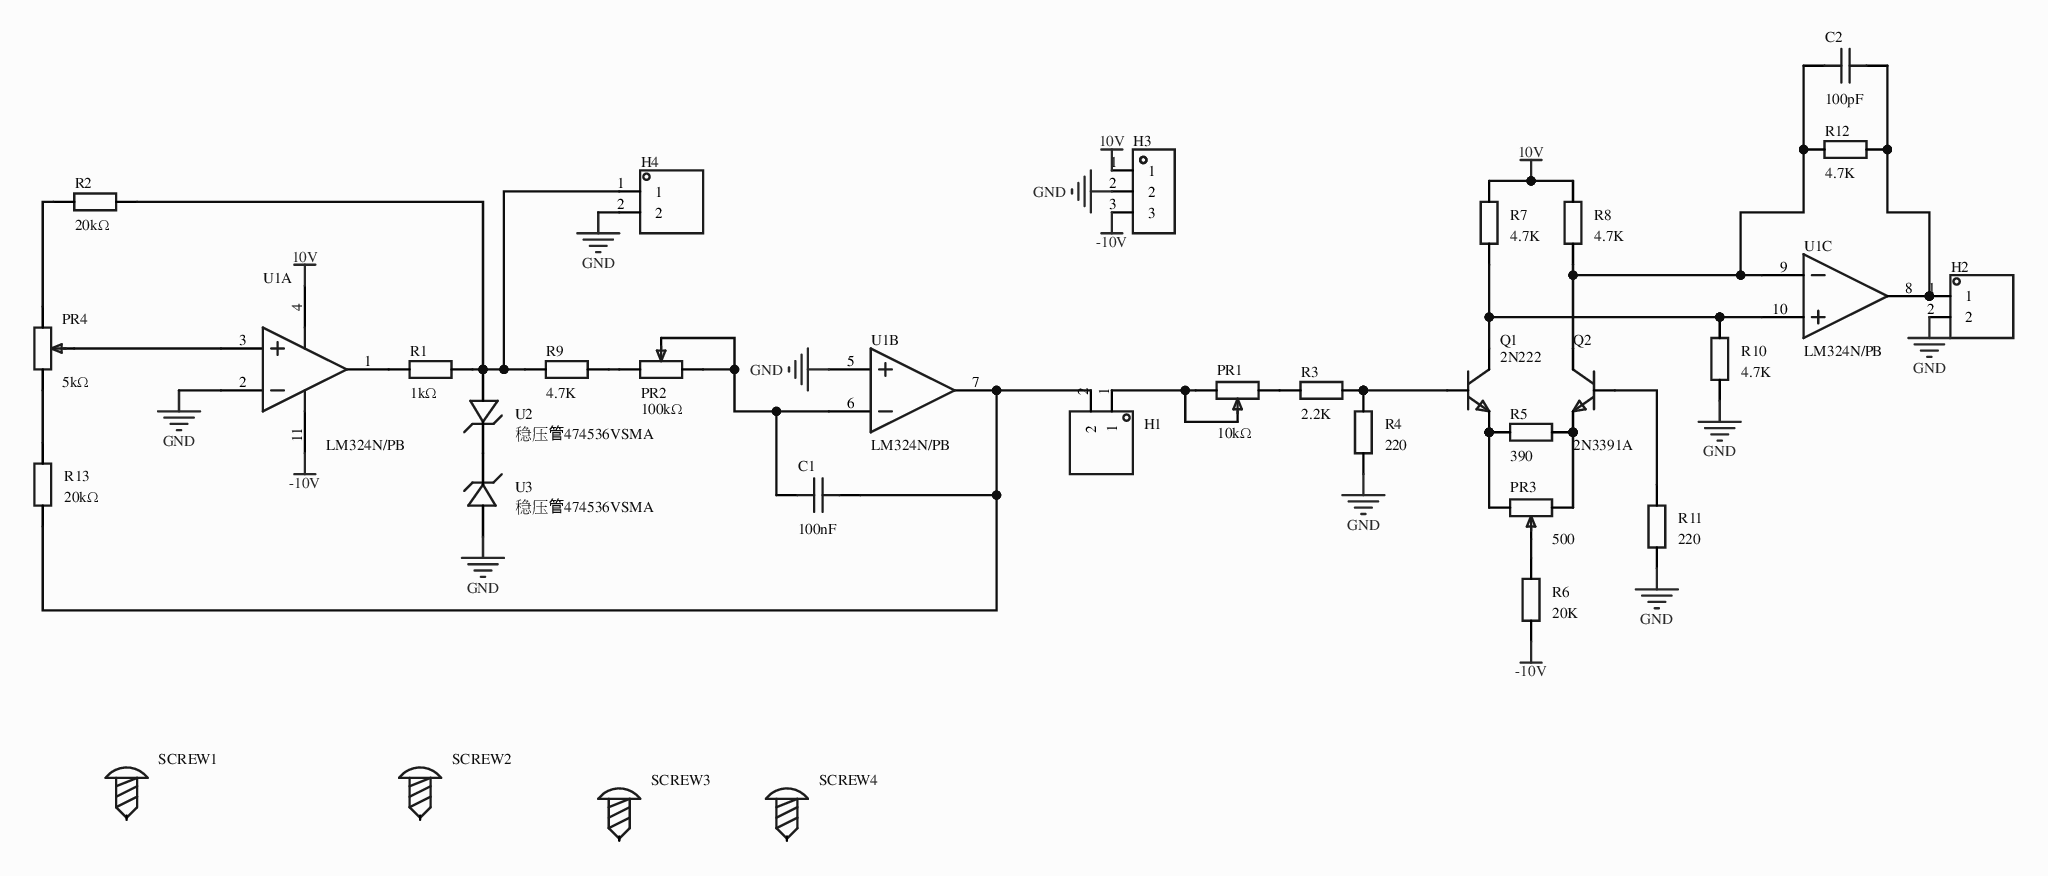
[diagram p0: MISC52119-3.schdoc]
# Altium project MISC52119-2.PrjPcb
1 sheet, 32 parts. Net scope: global (net labels, ports and power ports of the same name join across sheets).
Board file: MISC52119.pcbdoc

## Sheet MISC52119-3.schdoc
size 297 x 209 mm; Version: V1.0; @Project Name: MISC52119; @Update Date: 2026-03-23; @Create Date: 2026-03-23; @Board Name: MISC52119; @Create Time: 13:45:22; @Page Count: 1; @Page No: 1; @Schematic Name: MISC52119; @Update Time: 13:45:22; Size: A4

### Parts
C1  100nF  [C0603]
C2  100pF  [C0603]
H1  (no value)  [HDR-TH_2P-P2.54-V-M-1]
H2  (no value)  [HDR-TH_2P-P2.54-V-M-1]
H3  (no value)  [HDR-TH_3P-P2.54-V-M]
H4  (no value)  [HDR-TH_2P-P2.54-V-M-1]
PR1  10kΩ  [R_3296]
PR2  100kΩ  [R_3296]
PR3  500  [R_3296]
PR4  5kΩ  [R_3296]
Q1  2N222  [SMD_3-L3.0-W2.5_JANTXV2N2222AUB]
Q2  2N3391A  [TO-92-3_L4.9-W3.7-P1.27-L]
R1  1kΩ  [R0603]
R2  20kΩ  [R0603]
R3  2.2K  [R0603]
R4  220  [R0603]
R5  390  [R0603]
R6  20K  [R0603]
R7  4.7K  [R0603]
R8  4.7K  [R0603]
R9  4.7K  [R0603]
R10  4.7K  [R0603]
R11  220  [R0603]
R12  4.7K  [R0603]
R13  20kΩ  [R0603]
SCREW1  (no value)  [M2螺丝]
SCREW2  (no value)  [M2螺丝]
SCREW3  (no value)  [M2螺丝]
SCREW4  (no value)  [M2螺丝]
U1  LM324N/PB  [PDIP-14_L19.2-W6.6-P2.54-LS7.6-BL]  (parts A,B,C of 4)
U2  稳压管474536VSMA  [LL-41_L5.0-W2.5-RD]
U3  稳压管474536VSMA  [LL-41_L5.0-W2.5-RD]

### Nets
10V: H3.1 R7.2 R8.2 U1.4(V+)
-10V: H3.3 R6.1 U1.11(GND)
GND: H2.2 H3.2 H4.2 R4.1 R10.1 R11.1 U1.2(INA+) U1.5(INB+) U3.2(A)
NetC1_1: C1.1 H1.2 R13.2 U1.7(OUTB)
NetC1_2: C1.2 PR2.1 PR2.2 U1.6(INB-)
NetC2_1: C2.1 Q2.2(C) R8.1 R12.2 U1.9(INC-)
NetC2_2: C2.2 H2.1 R12.1 U1.8(OUTC)
NetH1_1: H1.1 PR1.1 PR1.2
NetH4_1: H4.1 R1.1 R2.1 R9.1 U2.2(A)
NetPR1_3: PR1.3 R3.1
NetPR2_3: PR2.3 R9.2
NetPR3_1: PR3.1 Q1.2(E) R5.1
NetPR3_2: PR3.2 R6.2
NetPR3_3: PR3.3 Q2.1(E) R5.2
NetPR4_1: PR4.1 R13.1
NetPR4_2: PR4.2 U1.3(INA-)
NetPR4_3: PR4.3 R2.2
NetQ1_1: Q1.1(C) R7.1 R10.2 U1.10(INC+)
NetQ1_3: Q1.3(B) R3.2 R4.2
NetQ2_3: Q2.3(B) R11.2
NetR1_2: R1.2 U1.1(OUTA)
NetU2_1: U2.1(C) U3.1(C)

Not connected (* = marked no-connect by the designer): SCREW1 1; SCREW2 1; SCREW3 1; SCREW4 1

### Library data of the parts
C1 C2 = CAP_0603: Symbol: Capacitance; 3D Model: ac125912035d415993ca9572d50418b10819f05c4eef4c71ace90d822a990e87; 3D Model Transform: 62.992,31.496,0,0,0,0,0,0,0; ConvertToPcb: yes; ModelName: C0603_L1.6-W0.8-H0.8; Device: CAP_0603; Supplier Footprint: 0603; AddInBom: yes; FootprintName: C0603
  C1: Value: 100nF
  C2: Value: 100pF
H1 H2 = HDR-M_2.54_1x2P: Symbol: 210S-1*2P L=11.6MMGold-plated black; 3D Model: 79b2e9f2d70a4d68a1b7098f27c6d4c50819f05c4eef4c71ace90d822a990e87; 3D Model Transform: 200,100,0,0,0,0,0,0,-118.11; ConvertToPcb: yes; ModelName: HDR-M-2.54_1x2; Device: HDR-M_2.54_1x2P; Supplier Part: C124375; Supplier Footprint: 插件; AddInBom: yes; FootprintName: HDR-TH_2P-P2.54-V-M-1
H3 = HDR-M_2.54_1x3P: 3D Model: bb473b6d38ff42a99216a4fcdbdcc4cb0819f05c4eef4c71ace90d822a990e87; 3D Model Transform: 300.03877,100,0,0,0,0,0,0,-118.11; AddInBom: yes; ModelName: HDR-TH_3P-P2.54-M-LI-1X3P; Symbol: HDR-M_2.54_1x3P; Device: HDR-M_2.54_1x3P; Supplier Part: C2937625; Supplier Footprint: 插件; ConvertToPcb: yes; FootprintName: HDR-TH_3P-P2.54-V-M
H4 = HDR-M_2.54_1x2P: Symbol: 210S-1*2P L=11.6MMGold-plated black; ConvertToPcb: yes; ModelId: 79b2e9f2d70a4d68a1b7098f27c6d4c50819f05c4eef4c71ace90d822a990e87; ModelName: HDR-M-2.54_1x2; ModelTransform: 200,100,0,0,0,0,0,0,-118.11; Device: HDR-M_2.54_1x2P; AddInBom: yes; SupplierPart: C124375; Supplier Footprint: 插件; FootprintName: HDR-TH_2P-P2.54-V-M-1
PR1 PR3 PR4 = R_3296: 3D Model: b182808559bb43bda9e7de64b64134cb0819f05c4eef4c71ace90d822a990e87; 3D Model Transform: 373.98,188.96,590.49,180,0,0,0,0,-140; ConvertToPcb: yes; ModelName: 3296W; Symbol: R_3296; Device: R_3296; Supplier Footprint: 直插; AddInBom: yes; FootprintName: R_3296
  PR1: Value: 10kΩ
  PR3: Value: 500
  PR4: Value: 5kΩ
PR2 = R_3296: ConvertToPcb: yes; ModelId: b182808559bb43bda9e7de64b64134cb0819f05c4eef4c71ace90d822a990e87; ModelName: 3296W; ModelTransform: 373.98,188.96,590.49,180,0,0,0,0,-140; Symbol: R_3296; Device: R_3296; Value: 100kΩ; AddInBom: yes; Supplier Footprint: 直插; FootprintName: R_3296
Q1 = JANTX2N2222AUB: 晶体管类型:NPN;集电极电流(Ic):800mA;集射极击穿电压(Vceo):50V;功率(Pd):500mW;直流电流增益(hFE@Ic,Vce):30@0.1mA,10V;; Manufacturer: MICROCHIP(美国微芯); AddInBom: yes; ModelId: 90bf7df7e71042edaee99df9cd0384ee0819f05c4eef4c71ace90d822a990e87; ModelTransform: 118.11,98.8187,0,0,0,0,0,0,0; Transistor Type: NPN; Collector Current (Ic): 800mA; Collector-Emitter Breakdown Voltage (Vceo): 50V; Power Dissipation (Pd): 500mW; Collector Cut-Off Current (Icbo): 10uA; Collector-Emitter Saturation Voltage (VCE(sat)@Ic,Ib): 300mV@150mA,15mA; Symbol: JANTX2N2222AUB; Device: JANTX2N2222AUB; Manufacturer Part: 2N222; LCSC Part Name: NPN 电流:800mA 耐压:50V; SupplierPart: C5658040; Supplier Footprint: SMD-3P; JLCPCB Part Class: Extended Part; Datasheet: https://atta.szlcsc.com/upload/public/pdf/source/20230606/E4E4BB560E81A9B18723DFB9400D168A.pdf; Supplier: LCSC; ConvertToPcb: yes; FootprintName: SMD_3-L3.0-W2.5_JANTXV2N2222AUB; ModelName: SMD_3-L3.0-W2.5_JANTXV2N2222AUB; DC Current Gain (hFE@Ic,Vce): 30@0.1mA,10V; Operating Temperature: -65℃~+200℃
Q2 = 2N3391A: 晶体管类型:NPN;集电极电流(Ic):500mA;集射极击穿电压(Vceo):25V;耗散功率(Pd):625mW;直流电流增益(hFE):250@2mA,4.5V;; Manufacturer: onsemi(安森美); AddInBom: yes; ModelId: aafe8e06f2154e7c93506efd0d6632dd0819f05c4eef4c71ace90d822a990e87; ModelTransform: 176.28752,144.88554,0,180,0,0,0,20.669,-196.85; type: NPN; Current - Collector(Ic): 500mA; Collector - Emitter Voltage VCEO: 25V; Pd - Power Dissipation(Pd): 625mW; Current - Collector Cutoff: 100nA; Symbol: 2N3391A; Device: 2N3391A; LCSC Part Name: 2N3391A; SupplierPart: C3201848; ManufacturerPart: 2N3391A; Supplier Footprint: TO-92-3; JLCPCB Part Class: Extended Part; Datasheet: https://atta.szlcsc.com/upload/public/pdf/source/20230915/95117444A113B71214574C7F553DD680.pdf; Supplier: LCSC; ConvertToPcb: yes; FootprintName: TO-92-3_L4.9-W3.7-P1.27-L; ModelName: TO-92-3_L4.9-W3.7-P1.27-L; DC Current Gain: 250@2mA,4.5V; Transition frequency(fT): -; Vce Saturation(VCE(sat)): -; Operating Temperature: -55℃~+150℃@(Tj)
R1 R3-R13 = Res_0603: Symbol: 电阻; 3D Model: fc143cca1e79419f9cd78b61e9279f080819f05c4eef4c71ace90d822a990e87; 3D Model Transform: 31.8897,63.7794,0,90,0,0,0,0,0; ConvertToPcb: yes; Device: Res_0603; Supplier Footprint: 0603; AddInBom: yes; FootprintName: R0603; ModelName: R0603
  R1: Value: 1kΩ
  R3: Value: 2.2K
  R4 R11: Value: 220
  R5: Value: 390
  R6: Value: 20K
  R7-R10 R12: Value: 4.7K
  R13: Value: 20kΩ
R2 = Res_0603: Symbol: 电阻; ConvertToPcb: yes; ModelId: fc143cca1e79419f9cd78b61e9279f080819f05c4eef4c71ace90d822a990e87; ModelTransform: 31.8897,63.7794,0,90,0,0,0,0,0; Device: Res_0603; Value: 20kΩ; AddInBom: yes; Supplier Footprint: 0603; FootprintName: R0603; ModelName: R0603
SCREW1-SCREW4 = M2螺丝: Symbol: 螺丝孔; ConvertToPcb: yes; Device: M2螺丝; AddInBom: yes; Supplier Footprint: 插件; FootprintName: M2螺丝
U1 = LM324N/PB: 放大器数:四路;增益带宽积(GBP):1MHz;输入偏置电流(Ib):45nA;; Manufacturer: TI(德州仪器); Relevance: []; AddInBom: yes; ModelId: 08aeb3774ab0450ba412f07c9830bd710819f05c4eef4c71ace90d822a990e87; ModelTransform: 755.904,309.842,0,0,0,0,0,0,-129.921; Number of Circuits: 四路; Gain Bandwidth Product(GBP): 1MHz; Current - Input Bias(Ib): 45nA; Output Current: 40mA; Symbol: LM324N/PB; Device: LM324N/PB; LCSC Part Name: LM324N/PB; SupplierPart: C4366406; ManufacturerPart: LM324N/PB; Supplier Footprint: PDIP-14; JLCPCB Part Class: Extended Part; Datasheet: https://atta.szlcsc.com/upload/public/pdf/source/20230921/264342EF71D0FEA3F079F4D0F511985F.pdf; Supplier: LCSC; ConvertToPcb: yes; FootprintName: PDIP-14_L19.2-W6.6-P2.54-LS7.6-BL; ModelName: PDIP-14_L19.2-W6.6-P2.54-LS7.6-BL; Operating Temperature: 0℃~+70℃
U2 U3 = 稳压管474536VSMA: AddInBom: yes; ModelId: cc8013af1bac4599ab3ed974f184204d0819f05c4eef4c71ace90d822a990e87; ModelName: LL-41_L5.0-W2.5; ModelTransform: 208.74,94.488,0,0,0,0,-0.005,0,0; Symbol: 稳压管474536VSMA; Device: 稳压管474536VSMA; LCSC Part Name: 稳压管474536VSMA; SupplierPart: C9900012221; ManufacturerPart: 稳压管474536VSMA; Supplier Footprint: LL-41; JLCPCB Part Class: Extended Part; Supplier: LCSC; ConvertToPcb: yes; FootprintName: LL-41_L5.0-W2.5-RD